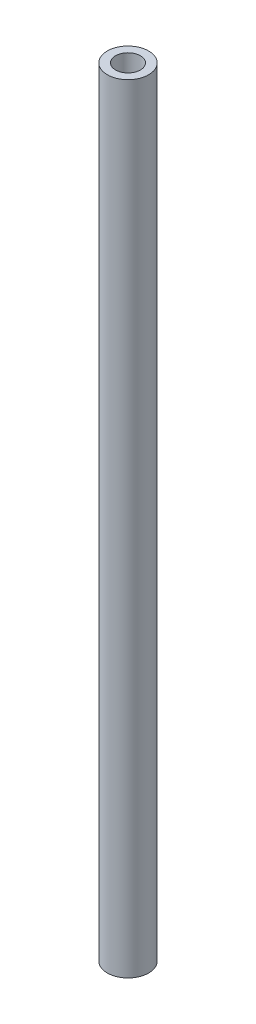
from build123d import *

# Parameters (mm, degrees)
SKETCH1_W = 0.2
SKETCH1_H = 18.84


with BuildPart() as part:
    # Sketch1 → Revolve2 (revolve)
    with BuildSketch(Plane.XY, mode=Mode.PRIVATE) as revolve2_sk:
        with Locations((-0.4, 9.42)):
            Rectangle(SKETCH1_W, SKETCH1_H)
    revolve(revolve2_sk.sketch.rotate(Axis((0, 23.646410138, 0), (0, -1, 0)), 270), axis=Axis((0, 23.646410138, 0), (0, -1, 0)))


solid = part.part
